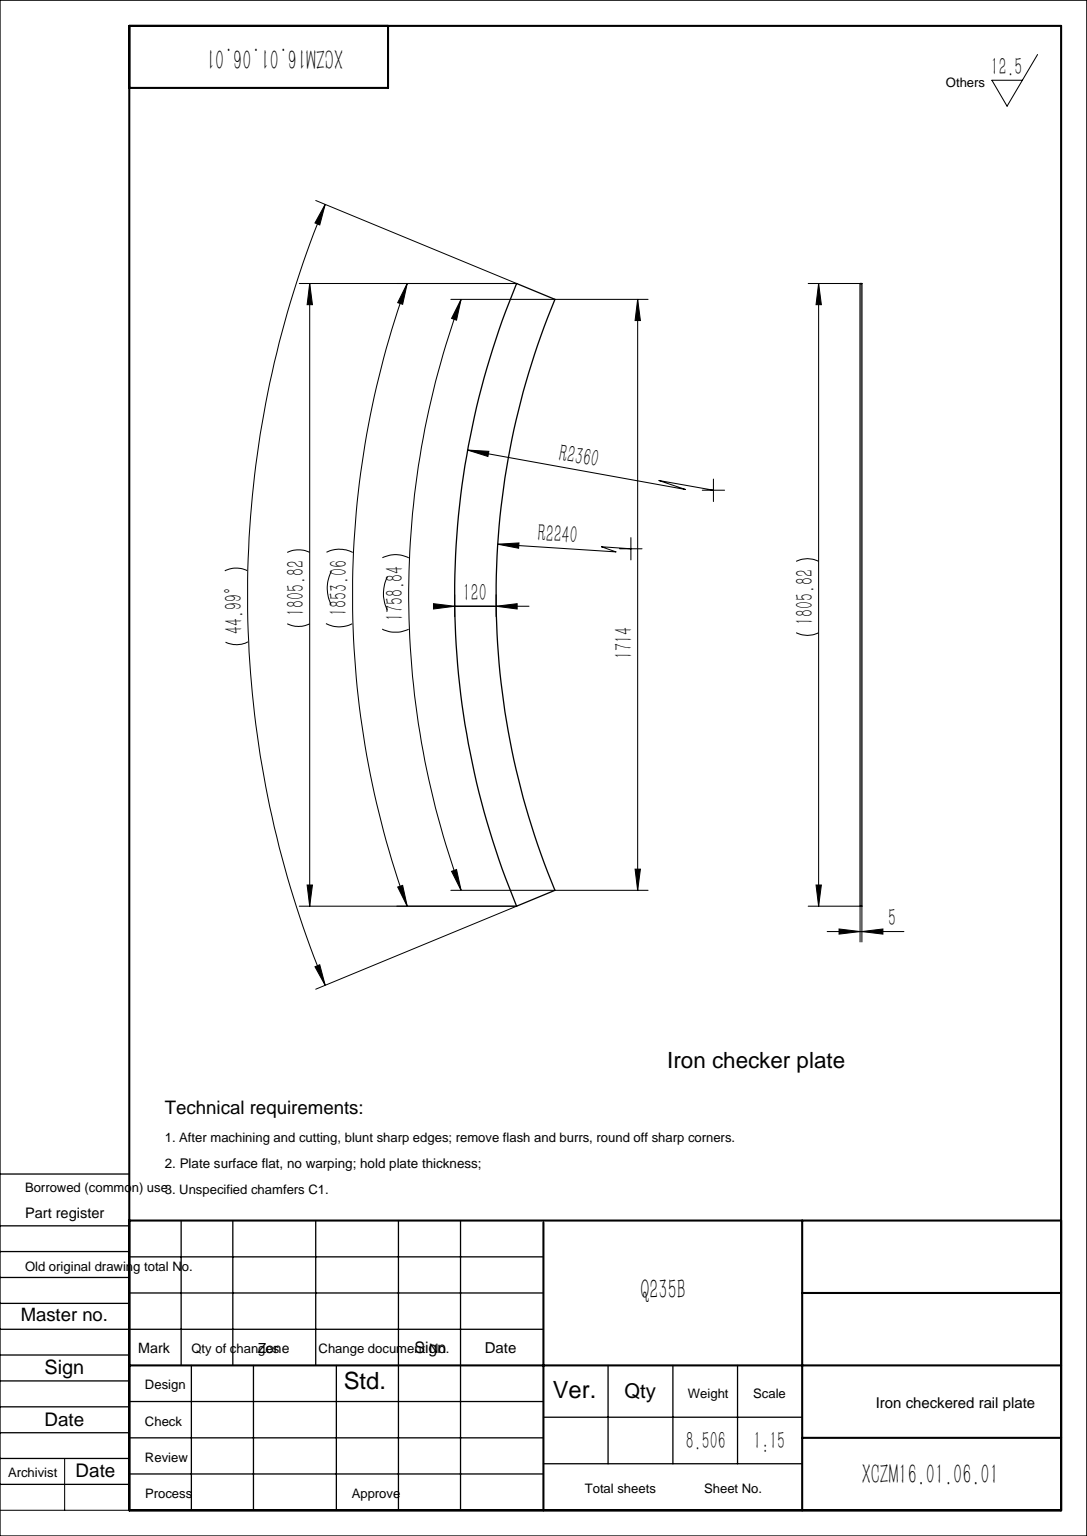
from build123d import *

# Parameters (mm, degrees)
BOSS_EXTRUDE1_DEPTH = 5


with BuildPart() as part:
    # Sketch2 → Boss-Extrude1 (new body)
    with BuildSketch(Plane(origin=(0, 0, 0), x_dir=(1, 0, 0), z_dir=(0, 1, 0))):
        with BuildLine():
            Line((-902.910714286, 2180.447715958), (-857, 2069.577493113))
            ThreePointArc((-857, 2069.577493113), (0, 2240), (857, 2069.577493113))
            Line((857, 2069.577493113), (902.910714286, 2180.447715958))
            ThreePointArc((902.910714286, 2180.447715958), (0, 2360), (-902.910714286, 2180.447715958))
        make_face()
    extrude(amount=BOSS_EXTRUDE1_DEPTH)


solid = part.part
